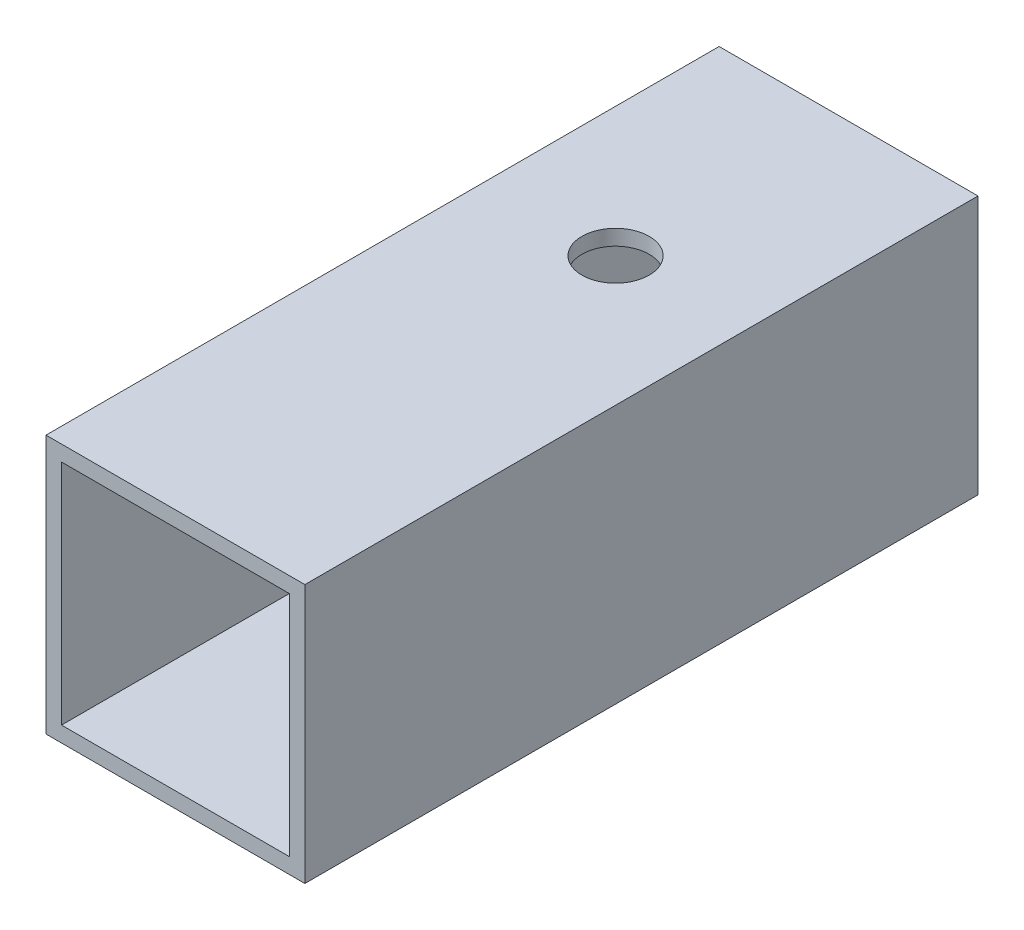
SolidWorks part; units mm, degrees
ref_plane "前视基准面" through (0, 0, 0) normal (0, 0, 1) x (1, 0, 0)
ref_plane "上视基准面" through (0, 0, 0) normal (0, 1, 0) x (1, 0, 0)
ref_plane "右视基准面" through (0, 0, 0) normal (1, 0, 0) x (0, 0, -1)
sketch "草图1" plane through (0, 0, 0) normal (0, 0, 1) x (1, 0, 0)
  line L0 (0, 0) -> (0, 50)
  line L1 (0, 50) -> (50, 50)
  line L2 (50, 50) -> (50, 0)
  line L3 (50, 0) -> (0, 0)
  line L4 (3, 3) -> (3, 47)
  line L5 (3, 47) -> (47, 47)
  line L6 (47, 47) -> (47, 3)
  line L7 (47, 3) -> (3, 3)
  dimension "D1" = 3
extrude "凸台-拉伸1" add sketch "草图1" along normal blind 130
sketch "草图4" plane through (0, 50, 0) normal (0, 1, 0) x (1, 0, 0)
  line L0 (25, 0) -> (25, -130)
  line L1 (50, 0) -> (0, 0) construction
  line L2 (50, -130) -> (0, -130) construction
sketch "草图5" plane through (0, 50, 0) normal (0, 1, 0) x (1, 0, 0)
  circle A0 centre (25, -45) radius 6.5
extrude "切除-拉伸1" cut sketch "草图5" against normal blind 130
sketch "草图6" plane through (50, 0, 0) normal (1, 0, 0) x (0, -1, 0)
  circle A0 centre (-60, -265) radius 6.5
